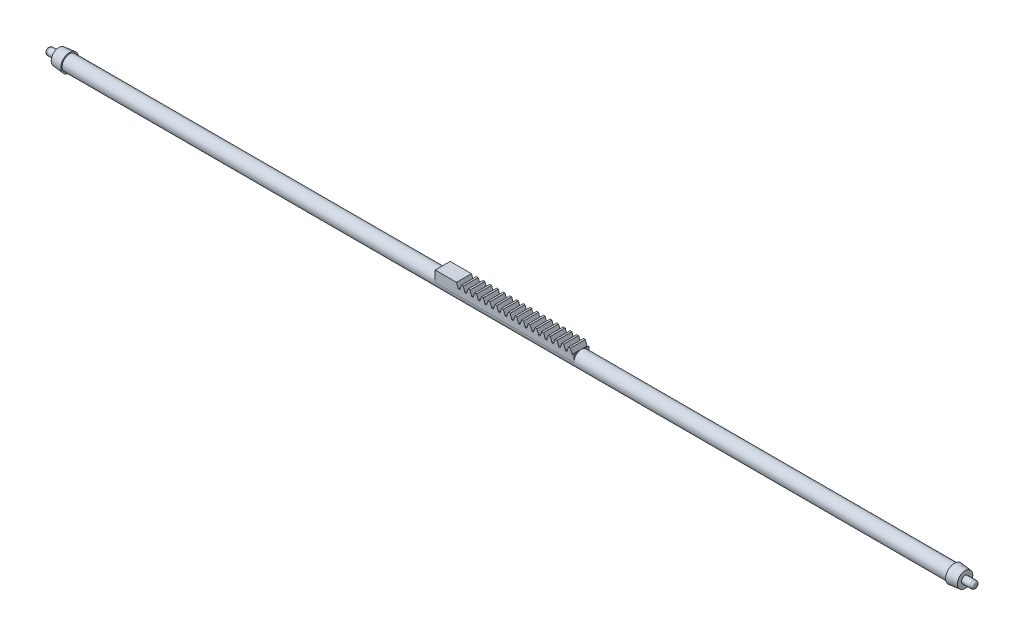
from build123d import *

# Parameters (mm, degrees)
SKETCH1_W            = 13
SKETCH1_H            = 1
BOSS_EXTRUDE1_DEPTH  = 1.4
CUT_EXTRUDE1_DEPTH   = 14.113351974
LPATTERN1_COUNT      = 18
LPATTERN1_PITCH      = 0.628
SKETCH3_R            = 0.7
BOSS_EXTRUDE2_DEPTH  = 35
BOSS_EXTRUDE3_START  = 13
BOSS_EXTRUDE3_DEPTH  = 13
BOSS_EXTRUDE4_START  = 35
SKETCH5_R            = 0.7
BOSS_EXTRUDE4_DEPTH  = 35
SKETCH6_R            = 0.829276609
BOSS_EXTRUDE5_DEPTH  = 1
BOSS_EXTRUDE5_TAPER  = 6
SKETCH7_R            = 0.329996585
BOSS_EXTRUDE6_DEPTH  = 1
FILLET1_R            = 0.2
FILLET1_OF_MIRROR1_R = 0.2


with BuildPart() as part:
    # Sketch1 → Boss-Extrude1 (new body)
    with BuildSketch(Plane.XY):
        with Locations((6.5, 0.5)):
            Rectangle(SKETCH1_W, SKETCH1_H)
    extrude(amount=BOSS_EXTRUDE1_DEPTH)

    # Sketch2 → Cut-Extrude1 (cut, through all)
    with BuildSketch(Plane.XY.offset(1.4)):
        Polygon((2, 1), (2.163786605, 0.55), (2.295961488, 0.55), (2.459748094, 1), align=None)
    cut_extrude1 = extrude(amount=-CUT_EXTRUDE1_DEPTH, mode=Mode.SUBTRACT)

    # LPattern1: Cut-Extrude1 ×18
    with Locations(*[(i * LPATTERN1_PITCH, 0, 0) for i in range(1, LPATTERN1_COUNT)]):
        add(cut_extrude1, mode=Mode.SUBTRACT)

    # Sketch3 → Boss-Extrude2 (add)
    with BuildSketch(Plane.ZY):
        with Locations((0.7, 0)):
            Circle(SKETCH3_R)
    extrude(amount=BOSS_EXTRUDE2_DEPTH)

    # Sketch4 → Boss-Extrude3 (add)
    with BuildSketch(Plane(origin=(0, 0, 0), x_dir=(0, 0, -1), z_dir=(1, 0, 0)).offset(BOSS_EXTRUDE3_START)):
        with BuildLine():
            Line((0, 0), (-1.4, 0))
            ThreePointArc((-1.4, 0), (-0.7, -0.7), (0, 0))
        make_face()
    extrude(amount=-BOSS_EXTRUDE3_DEPTH)

    # Sketch5 → Boss-Extrude4 (add)
    with BuildSketch(Plane(origin=(13, 0, 0), x_dir=(0, 0, -1), z_dir=(1, 0, 0)).offset(BOSS_EXTRUDE4_START)):
        with Locations((-0.7, 0)):
            Circle(SKETCH5_R)
    extrude(amount=-BOSS_EXTRUDE4_DEPTH)

    # Sketch6 → Boss-Extrude5 (add)
    with BuildSketch(Plane(origin=(48, 0, 0), x_dir=(0, 0, -1), z_dir=(1, 0, 0))):
        with Locations((-0.7, 0)):
            Circle(SKETCH6_R)
    boss_extrude5 = extrude(amount=BOSS_EXTRUDE5_DEPTH, taper=BOSS_EXTRUDE5_TAPER)

    # Sketch7 → Boss-Extrude6 (add)
    with BuildSketch(Plane(origin=(49, 0, 0), x_dir=(0, 0, -1), z_dir=(1, 0, 0))):
        with Locations((-0.7, 0)):
            Circle(SKETCH7_R)
    boss_extrude6 = extrude(amount=BOSS_EXTRUDE6_DEPTH)

    # Fillet1
    fillet1_edges = [part.edges().sort_by_distance(p)[0] for p in [
        (50, 0, 1.029996585),
    ]]
    fillet(fillet1_edges, radius=FILLET1_R)

    # Mirror1: Boss-Extrude5, Boss-Extrude6 across plane
    add(boss_extrude5.mirror(Plane.ZY.offset(-6.5)))
    add(boss_extrude6.mirror(Plane.ZY.offset(-6.5)))

    # Fillet1 of Mirror1
    fillet1_of_mirror1_edges = [part.edges().sort_by_distance(p)[0] for p in [
        (-37, 0, 1.029996585),
    ]]
    fillet(fillet1_of_mirror1_edges, radius=FILLET1_OF_MIRROR1_R)


solid = part.part
